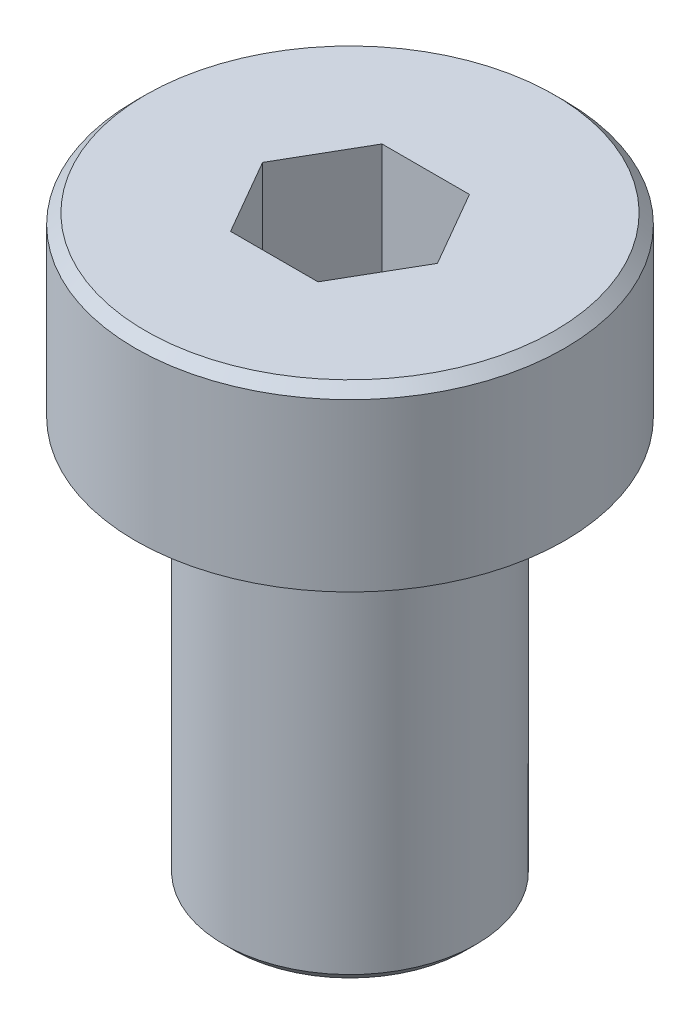
from build123d import *

# Parameters (mm, degrees)
CHAMFER1_SIZE         = 0.2
CUT_EXTRUDE1_DEPTH    = 2.7
BODY_MOVE_COPY1_ANGLE = 180


with BuildPart() as part:
    # Sketch2 → Revolve1 (revolve)
    with BuildSketch(Plane.XY):
        Polygon((1.5, -3.5), (1.5, -0.8), (0, 0.066025404), (0, 8), (2.5, 8), (2.5, 0), (4.25, 0), (4.25, -3.5), align=None)
    revolve(axis=Axis((0, 0.066025404, 0), (0, 1, 0)))

    # Chamfer1
    chamfer1_edges = [part.edges().sort_by_distance(p)[0] for p in [
        (-4.25, -3.5, 0),
        (-2.5, 8, 0),
    ]]
    chamfer(chamfer1_edges, length=CHAMFER1_SIZE)

    # Sketch3 → Cut-Extrude1 (cut)
    with BuildSketch(Plane.XZ.offset(3.5)):
        Polygon((-0.866025404, 1.5), (-1.732050808, 0), (-0.866025404, -1.5), (0.866025404, -1.5), (1.732050808, 0), (0.866025404, 1.5), align=None)
    extrude(amount=-CUT_EXTRUDE1_DEPTH, mode=Mode.SUBTRACT)


with BuildPart() as part_1:
    # Body-Move/Copy1: moved
    add(part.part.rotate(Axis((0, 3.25, 0), (1, 0, 0)), BODY_MOVE_COPY1_ANGLE))


solid = part_1.part
